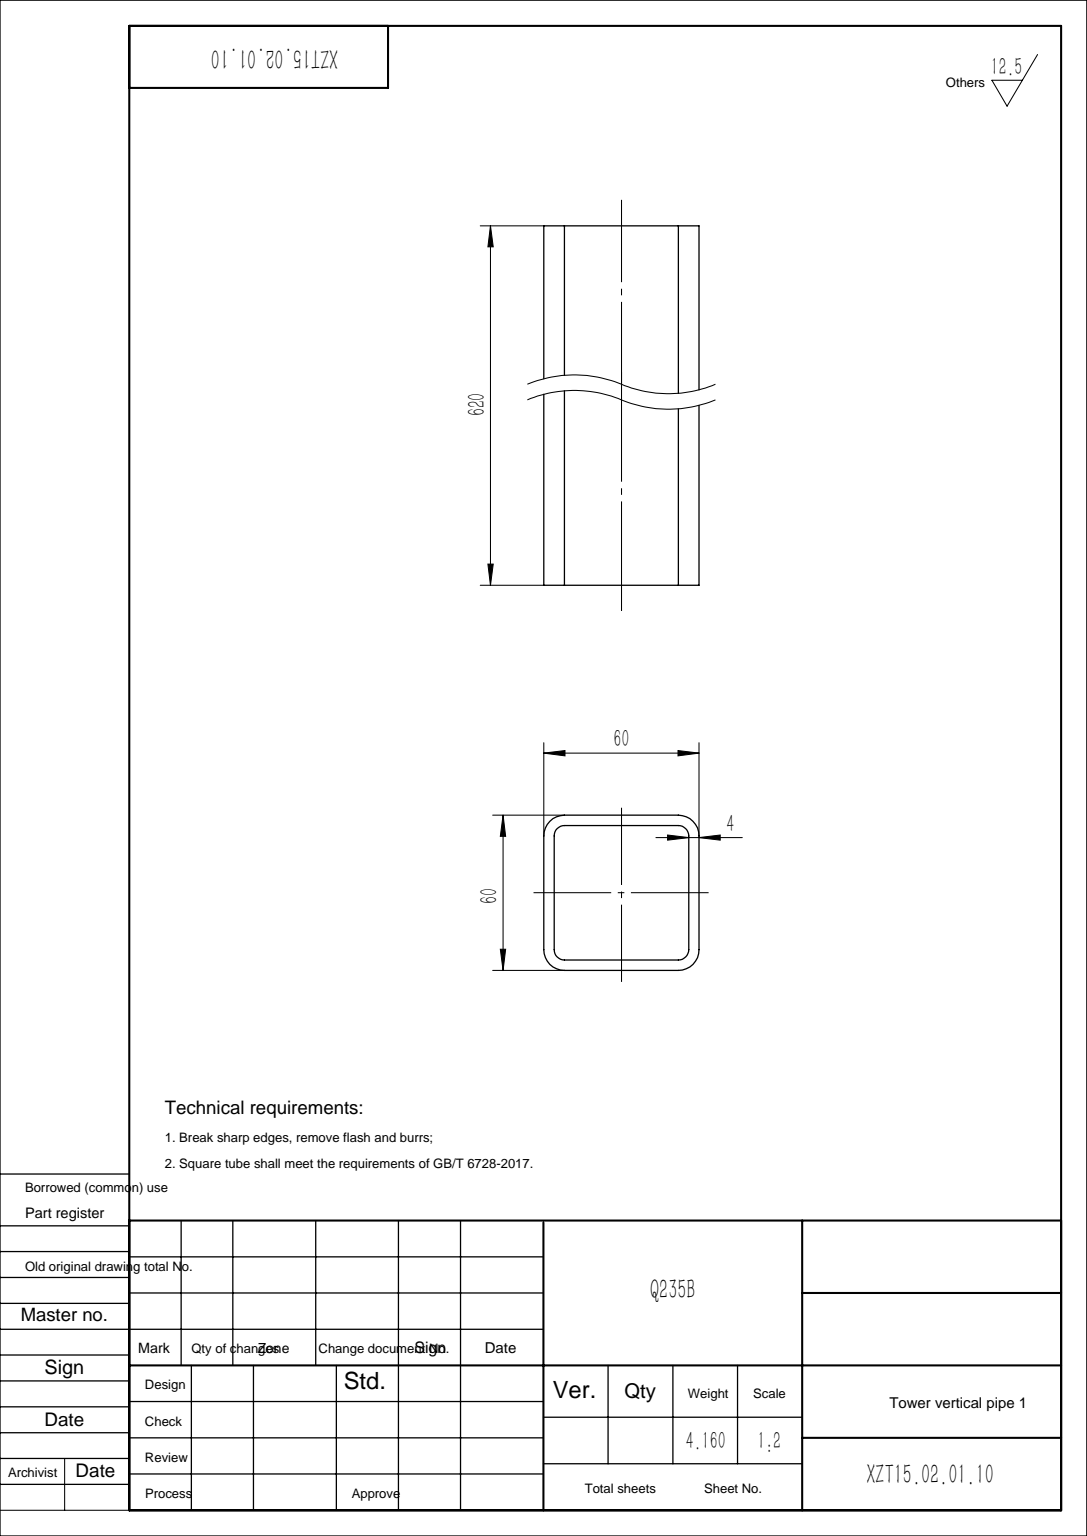
SolidWorks part; units mm, degrees
material "Q235B"
ref_plane "Front Plane" through (0, 0, 0) normal (0, 0, 1) x (1, 0, 0)
ref_plane "Top Plane" through (0, 0, 0) normal (0, 1, 0) x (1, 0, 0)
ref_plane "Right Plane" through (0, 0, 0) normal (1, 0, 0) x (0, 0, -1)
sketch "草图1" plane through (0, 0, 0) normal (0, 0, 1) x (1, 0, 0)
  line L0 (0, 0) -> (0, 620)
  dimension "D1" = 620
other "GB/T 6728-2002 square hollow section 60×60×4(1)"
ref_plane "Plane1" through (0, 0, 0) normal (0, 1, 0) x (-1, 0, 0)
sketch "Sketch1" plane through (0, 0, 0) normal (0, 1, 0) x (-1, 0, 0)
  line L0 (-22, -26) -> (22, -26)
  line L1 (-26, -22) -> (-26, 22)
  line L2 (22, 26) -> (-22, 26)
  line L3 (26, 22) -> (26, -22)
  line L4 (-22, -30) -> (22, -30)
  line L5 (-30, -22) -> (-30, 22)
  line L6 (22, 30) -> (-22, 30)
  line L7 (30, 22) -> (30, -22)
  arc A0 (30, 22) -> (22, 30) centre (22, 22) ccw
  arc A1 (22, -30) -> (30, -22) centre (22, -22) ccw
  arc A2 (-30, -22) -> (-22, -30) centre (-22, -22) ccw
  arc A3 (-22, 30) -> (-30, 22) centre (-22, 22) ccw
  arc A4 (-22, 26) -> (-26, 22) centre (-22, 22) ccw
  arc A5 (26, 22) -> (22, 26) centre (22, 22) ccw
  arc A6 (22, -26) -> (26, -22) centre (22, -22) ccw
  arc A7 (-26, -22) -> (-22, -26) centre (-22, -22) ccw
  point P0 (-30, 0)
  point P1 (30, 0)
  point P2 (0, 30)
  point P3 (0, -30)
  point P4 (0, 0)
  point P5 (-30, -30)
  point P6 (30, -30)
  point P7 (30, 30)
  point P8 (-30, 30)
  point P33 (0, 0)
  dimension "D1" = 8
  dimension "Thickness" = 4
  dimension "V_leg" = 60
